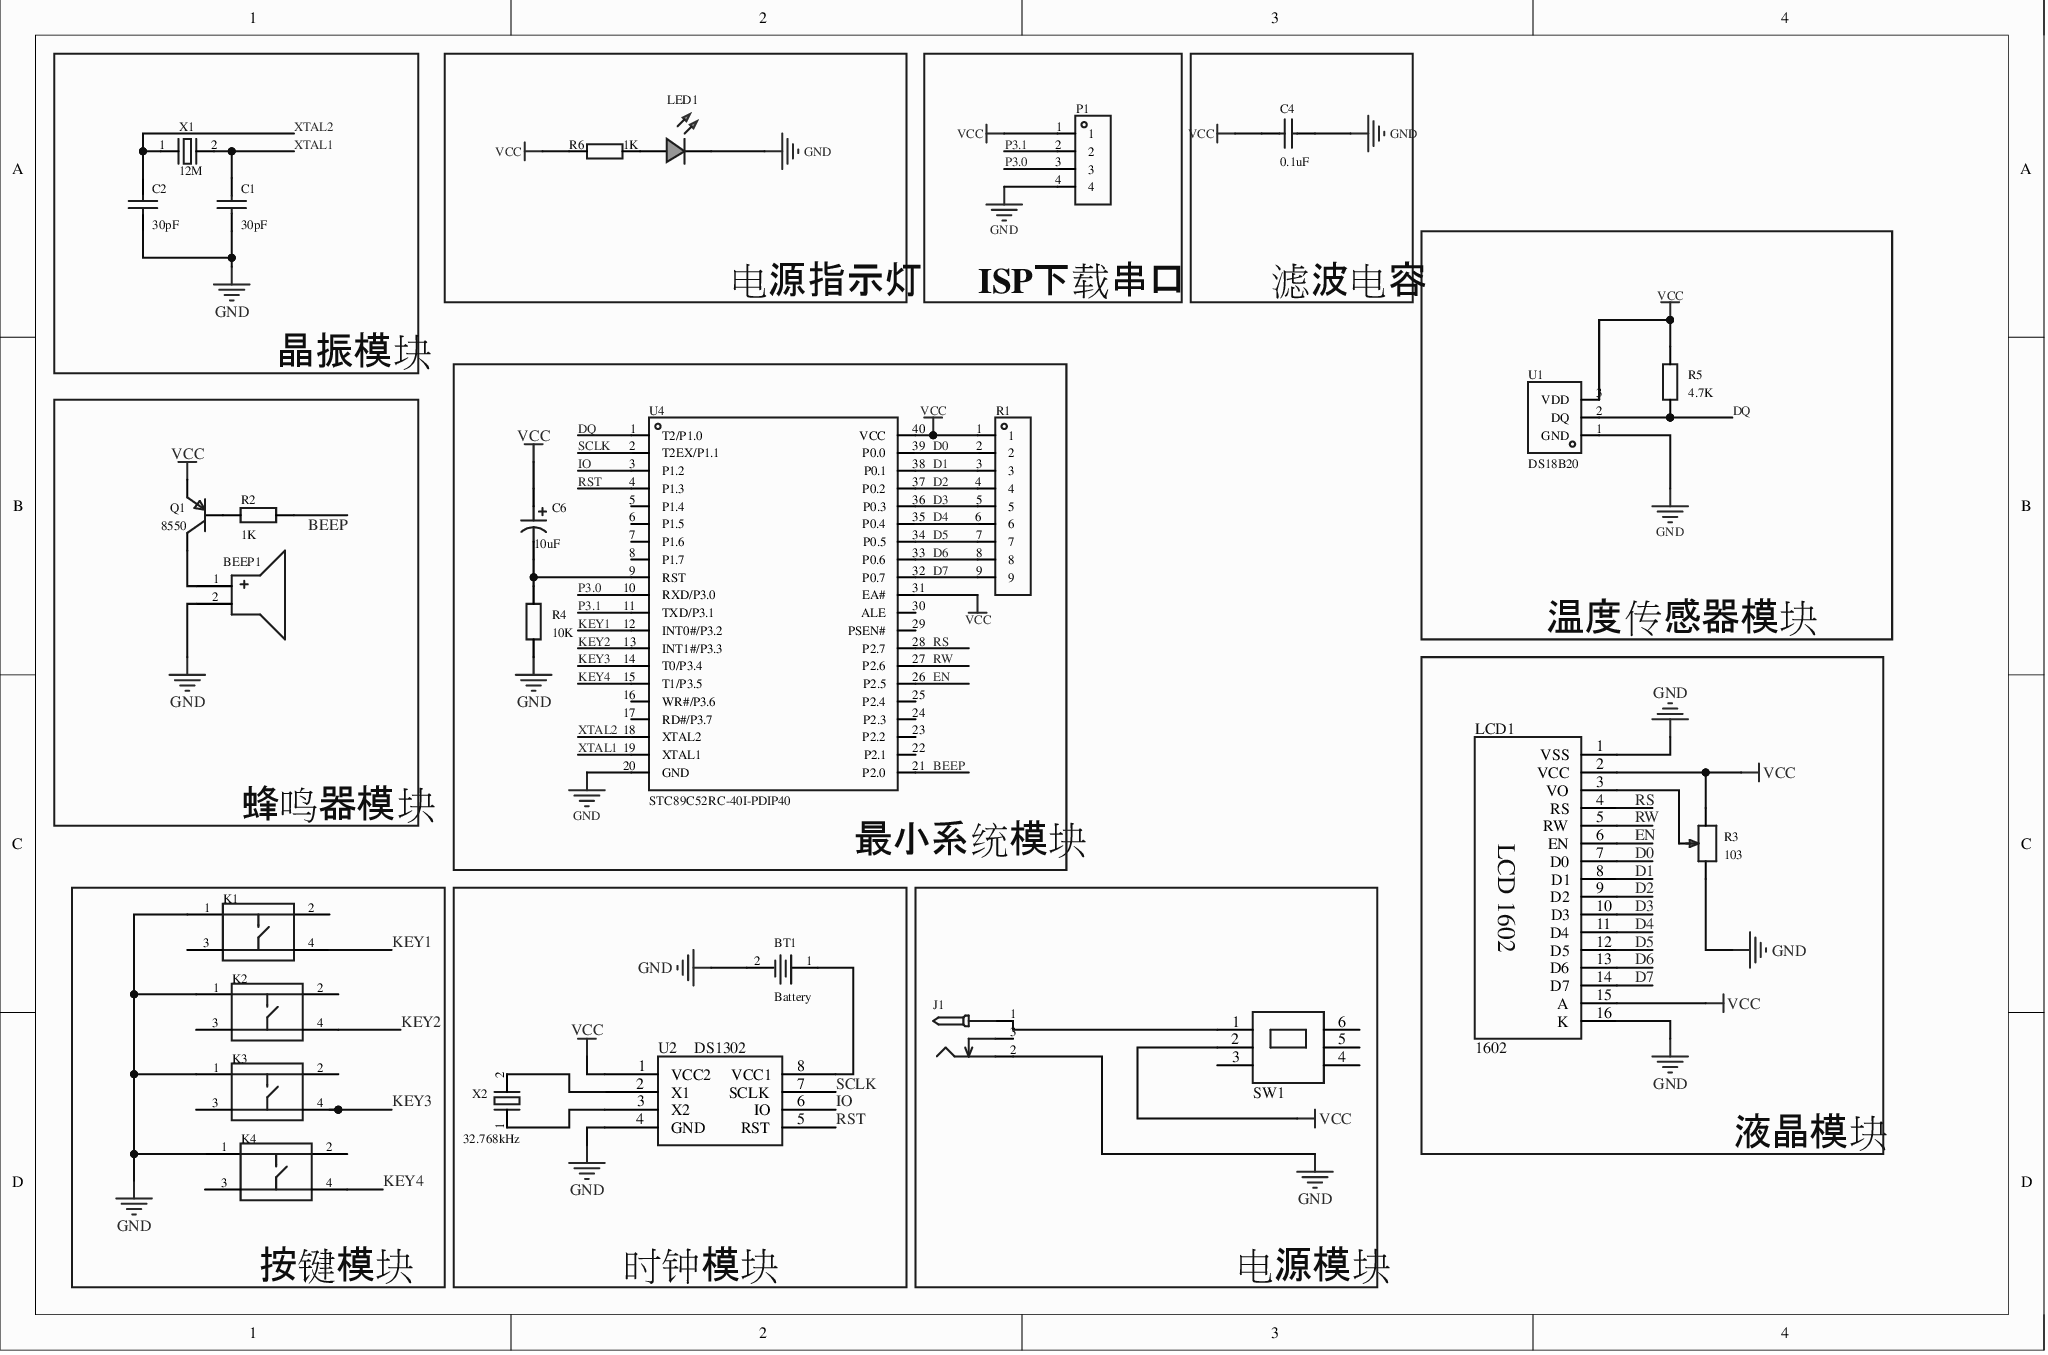
[diagram p0: MISC51236-2.schdoc]
# Altium project MISC51236-3.PrjPcb
1 sheet, 27 parts. Net scope: global (net labels, ports and power ports of the same name join across sheets).
Board file: MISC51236.pcbdoc

## Sheet MISC51236-2.schdoc
size 292 x 193 mm; Name: MISC51236

### Parts
BEEP1  (no value)  [BUZ-TH_BD12.0-P7.60-D0.6-FD]
BT1  Battery  [BAT-TH_CR2032]
C1  30pF  [CAP-TH_L5.0-W4.0-P5.00-D1.0]
C2  30pF  [CAP-TH_L5.0-W4.0-P5.00-D1.0]
C4  0.1uF  [CAP-TH_L5.0-W4.0-P5.00-D1.0]
C6  10uF  [CAP-TH_BD5.0-P2.00-D0.6-FD]
J1  (no value)  [DC-005_2.5]
K1  (no value)  [KEY-TH_4P-L6.0-W6.0-P4.50-LS6.50]
K2  (no value)  [KEY-TH_4P-L6.0-W6.0-P4.50-LS6.50]
K3  (no value)  [KEY-TH_4P-L6.0-W6.0-P4.50-LS6.50]
K4  (no value)  [KEY-TH_4P-L6.0-W6.0-P4.50-LS6.50]
LCD1  1602  [HDR-M-2.54_1X16]
LED1  (no value)  [LED-TH_5mm]
P1  (no value)  [HDR-TH_4P-P2.54-V-M]
Q1  8550  [S8550P_TO-92]
R1  (no value)  [SIP-9_L22.3-W3.2-P2.54_KA2284-SIP-9]
R2  1K  [Res_1/4W]
R3  103  [RES-ADJ-SMD_RM065-V1]
R4  10K  [Res_1/4W]
R5  4.7K  [Res_1/4W]
R6  1K  [Res_1/4W]
SW1  SWT  [SW-TH_6P-L8.5-W8.5-P2.50-LS5.5-BL-2]  (value not drawn)
U1  DS18B20  [TO-92-3_L4.5-W3.5-P1.27-L]
U2  DS1302  [DIP-8_L10.9-W6.4-P2.54-LS7.6-BL]
U4  STC89C52RC-40I-PDIP40  [DIP-40_L52.0-W13.7-P2.54-LS15.2-BL]
X1  12M  [HC-49S_L11.5-W4.7-P4.88]
X2  32.768kHz  [XTAL2]

### Blocks framed on the sheet
晶振模块: C1 C2 X1
电源指示灯: LED1 R6
ISP下载串口: P1
滤波电容: C4
温度传感器模块: R5 U1
最小系统模块: C6 R1 R4 U4
蜂鸣器模块: BEEP1 Q1 R2
液晶模块: LCD1 R3
按键模块: K1-K4
时钟模块: BT1 U2 X2
电源模块: J1 SW1

### Nets
GND: BEEP1.2(-) BT1.2 C1.1 C2.1 C4.2 J1.2 K1.1 K2.1 K3.1 K4.1 LCD1.1(VSS) LCD1.16(K) LED1.2(A) P1.4 R3.1 R4.1 U1.1(GND) U2.4(GND) U4.20(GND)
VCC: C4.1 C6.1 LCD1.2(VCC) LCD1.15(A) P1.1 Q1.1(E) R1.1 R3.3 R5.2 R6.1 SW1.2 U1.3(VDD) U2.1(VCC2) U4.31(EA#) U4.40(VCC)
BEEP: R2.2 U4.21(P2.0)
D0: LCD1.7(D0) R1.2 U4.39(P0.0)
D1: LCD1.8(D1) R1.3 U4.38(P0.1)
D2: LCD1.9(D2) R1.4 U4.37(P0.2)
D3: LCD1.10(D3) R1.5 U4.36(P0.3)
D4: LCD1.11(D4) R1.6 U4.35(P0.4)
D5: LCD1.12(D5) R1.7 U4.34(P0.5)
D6: LCD1.13(D6) R1.8 U4.33(P0.6)
D7: LCD1.14(D7) R1.9 U4.32(P0.7)
DQ: R5.1 U1.2(DQ) U4.1(T2/P1.0)
EN: LCD1.6(EN) U4.26(P2.5)
IO: U2.6(IO) U4.3(P1.2)
KEY1: K1.4 U4.12(INT0#/P3.2)
KEY2: K2.4 U4.13(INT1#/P3.3)
KEY3: K3.4 U4.14(T0/P3.4)
KEY4: K4.4 U4.15(T1/P3.5)
P3.0: P1.3 U4.10(RXD/P3.0)
P3.1: P1.2 U4.11(TXD/P3.1)
RS: LCD1.4(RS) U4.28(P2.7)
RST: U2.5(RST) U4.4(P1.3)
RW: LCD1.5(RW) U4.27(P2.6)
SCLK: U2.7(SCLK) U4.2(T2EX/P1.1)
XTAL1: C1.2 U4.19(XTAL1) X1.2
XTAL2: C2.2 U4.18(XTAL2) X1.1
NetBEEP1_1: BEEP1.1(+) Q1.3(C)
NetBT1_1: BT1.1 U2.8(VCC1)
NetC6_2: C6.2 R4.2 U4.9(RST)
NetJ1_1: J1.1 SW1.1
NetLCD1_3: LCD1.3(VO) R3.2
NetLED1_1: LED1.1(C) R6.2
NetQ1_2: Q1.2(B) R2.1
NetU2_2: U2.2(X1) X2.2
NetU2_3: U2.3(X2) X2.1

Not connected (* = marked no-connect by the designer): J1 3*; K1 2* 3*; K2 2* 3*; K3 2* 3*; K4 2* 3*; SW1 3(2)* 4(3)* 5(4)* 6(5)*; U4 5(P1.4)* 6(P1.5)* 7(P1.6)* 8(P1.7)* 16(WR#/P3.6)* 17(RD#/P3.7)* 22(P2.1)* 23(P2.2)* 24(P2.3)* 25(P2.4)* 29(PSEN#)* 30(ALE)*

### Library data of the parts
BEEP1 = BZ-D12-L7_6: AddInBom: yes; ModelId: 16ab50e14c5b4f2c986c135bdba60e370819f05c4eef4c71ace90d822a990e87; ModelName: BUZ-TH_D12.0-H9.5-P7.60; ModelTransform: 472.44,472.176,0,90,0,0,-0.787,0,-177.165; Symbol: BZ-D12-L7_6; Device: BZ-D12-L7_6; LCSC Part Name: BZ-D12-L7_6; SupplierPart: C9900009978; Supplier Footprint: BUZ-TH; JLCPCB Part Class: Extended Part; Supplier: LCSC; ConvertToPcb: yes; FootprintName: BUZ-TH_BD12.0-P7.60-D0.6-FD
BT1 = Q&J CR2032 20-6*9_C9900112302: AddInBom: yes; ModelId: 2a22c62c6e424c70bca0a6138eddf4b70819f05c4eef4c71ace90d822a990e87; ModelTransform: 814.959,786.69055,0,180,0,0,0,0,-196.85; Symbol: Q&J CR2032 20-6*9; Device: Q&J CR2032 20-6*9_C9900112302; Manufacturer Part: Battery; LCSC Part Name: Q&J CR2032 20-6*9; SupplierPart: C9900112302; Supplier Footprint: BAT-TH_CR2032; JLCPCB Part Class: Extended Part; Supplier: LCSC; ConvertToPcb: yes; FootprintName: BAT-TH_CR2032; ModelName: BAT-TH_CR2032
C1 C2 C4 = 瓷片电容47PF 3KV: 容值:-;额定电压:-;温度系数:-;; Symbol: Ceramic capacitors47PF 3KV; AddInBom: yes; ModelId: 7562e8dfad8b481384451709c5473ca60819f05c4eef4c71ace90d822a990e87; ModelName: CAP-TH_BD5.0-W4.0-P5.08; ModelTransform: 224.49711,157.48,0,0,0,0,0,0,-137.795; Device: 瓷片电容47PF 3KV; LCSC Part Name: 47pF(47R) ±10% 3KV; ManufacturerPart: 瓷片电容47PF 3KV; Supplier Footprint: 插件; JLCPCB Part Class: Extended Part; Supplier: LCSC; ConvertToPcb: yes; FootprintName: CAP-TH_L5.0-W4.0-P5.00-D1.0; Voltage Rated: -; Lead Spacing: -; Temperature Coefficient: -; φD: -; Body Thickness: -
  C1 C2: Value: 30pF
  C4: Value: 0.1uF
C6 = 10uF/25V-C5X11DIP: AddInBom: yes; ModelId: e14933aa819f4e768454ffe1b66cd5400819f05c4eef4c71ace90d822a990e87; ModelTransform: 196.70055,196.77528,0,0,0,0,0.118,0,-137.795; Symbol: 10UF/25V-C5X11DIP; Device: 10uF/25V-C5X11DIP; Manufacturer Part: 10uF; LCSC Part Name: 10uF/25V-C5X11DIP; SupplierPart: C9900003841; Supplier Footprint: CAP-TH_BD5.0-P2.00; JLCPCB Part Class: Extended Part; Supplier: LCSC; ConvertToPcb: yes; FootprintName: CAP-TH_BD5.0-P2.00-D0.6-FD; ModelName: CAP-TH_BD5.0-P2.00-D0.6-FD
J1 = DC-005_2.5: ConvertToPcb: yes; ModelId: f168fe383f964e0ea2af0127ff6ac7b40819f05c4eef4c71ace90d822a990e87; ModelName: DC-IN-TH_DC005; ModelTransform: 366.14,553.15,590.55,90,0,0,137.8,-11.81,-157.48; Symbol: DC-005_2.5; Device: DC-005_2.5; AddInBom: yes; Supplier Footprint: 插件; FootprintName: DC-005_2.5
K1-K4 = K2-1102DP-C4SW-04: 电路结构:单刀单掷;按钮形状:圆形按钮;作用力:2.5N;安装方式:直插;开关长度:6mm;开关宽度:6mm;开关高度:5mm;触点电流:50mA;额定电压:12V;带灯:-;工作寿命:10万次;; Manufacturer: 韩国韩荣; AddInBom: yes; ModelId: b38fea4b2e4e408486f1d54ff7bc5cc00819f05c4eef4c71ace90d822a990e87; ModelTransform: 307.086,236.22,0,0,0,0,0,0,-137.795; Circuit: 单刀单掷; Actuator Style: 圆形按钮; Operating Force: 2.5N; Switch Height: 5mm; Contact Current: 50mA; Voltage Rating: 12V; Life: 10万次; Symbol: K2-1102DP-C4SW-04; Device: K2-1102DP-C4SW-04; LCSC Part Name: 轻触按键开关6*6*5; SupplierPart: C110153; Supplier Footprint: 插件-4P,6x6mm; JLCPCB Part Class: Extended Part; Datasheet: https://item.szlcsc.com/datasheet/K2-1102DP-C4SW-04/111374.html; Supplier: LCSC; ConvertToPcb: yes; FootprintName: KEY-TH_4P-L6.0-W6.0-P4.50-LS6.50; ModelName: KEY-TH_4P-L6.0-W6.0-P4.50-LS6.50; Mounting Type: 直插; Length: 6mm; Width: 6mm; With Lamp: -; Operating Temperature: -25℃~+85℃
LCD1 = 1602_1: AddInBom: yes; Device: 1602_1; DesignItemID: 1602; LibraryName: MANUAL; Symbol: 1602; FootprintName: HDR-M-2.54_1X16
LED1 = LED_TH-G_5mm: ConvertToPcb: yes; ModelId: fe7796f666a04da4b4289311169b45200819f05c4eef4c71ace90d822a990e87; ModelName: LED-TH_BD5.8-P2.54-FD_GREEN-1; ModelTransform: 212.58,227.91,537.36,0,0,0,-7.87,0,-196.85; Symbol: LED_TH-G; Device: LED_TH-G_5mm; AddInBom: yes; Supplier Footprint: 插件; FootprintName: LED-TH_5mm
P1 = HDR-M_2.54_1x4P: Symbol: PZ254V-11-04P; ConvertToPcb: yes; ModelId: 112f4d05e8d64e99ab9a333894bea4f90819f05c4eef4c71ace90d822a990e87; ModelName: HDR-TH_4P-P2.54-M-LI-1X4P; ModelTransform: 399.999,104.7242,0,0,0,0,0,0,-118.11; Device: HDR-M_2.54_1x4P; AddInBom: yes; SupplierPart: C492403; Supplier Footprint: 插件; FootprintName: HDR-TH_4P-P2.54-V-M
Q1 = S8550_TO_PNP: ConvertToPcb: yes; ModelId: aafe8e06f2154e7c93506efd0d6632dd0819f05c4eef4c71ace90d822a990e87; ModelName: TO-92-3_L4.9-W3.7-P1.27-L; ModelTransform: 180.78,141.44,417.3,0,0,0,0,0,-200; Symbol: S8550_TO_PNP; Device: S8550_TO_PNP; AddInBom: yes; Supplier Footprint: TO-92; FootprintName: S8550P_TO-92
R1 = HDR-M_2.54-1x9P: Symbol: PZ254V-11-09P; 3D Model: b5c1e988b3bb4503807579736b357ad00819f05c4eef4c71ace90d822a990e87; 3D Model Transform: 890.15562,98.425,0,0,0,0,0,0,-118.11; ConvertToPcb: yes; ModelName: HDR-TH_9P-P2.54-M-LI-1X9P; Device: HDR-M_2.54-1x9P; Supplier Part: C492408; Supplier Footprint: 插件; AddInBom: yes; FootprintName: SIP-9_L22.3-W3.2-P2.54_KA2284-SIP-9
R2 R4-R6 = Res_AXIAL-1/4W: Symbol: 电阻; 3D Model: 463263665006444ab7a47bd11b0cf9560819f05c4eef4c71ace90d822a990e87; 3D Model Transform: 427.165,94.32816,0,0,0,0,0,0,-196.85; AddInBom: yes; ModelName: RES-TH_BD2.4-L6.3-P10.30-D0.6; Device: Res_AXIAL-1/4W; Supplier Footprint: 轴向引线; ConvertToPcb: yes; FootprintName: Res_1/4W
  R2 R6: Value: 1K
  R4: Value: 10K
  R5: Value: 4.7K
R3 = RM065-V1-103: AddInBom: yes; ModelId: c816c2b7942147f5a832150e8ef6960c0819f05c4eef4c71ace90d822a990e87; ModelTransform: 255.905,283.464,0,0,0,0,0.025,-3.937,-157.48; Symbol: RM065-V1-103; Device: RM065-V1-103; Manufacturer Part: 103; LCSC Part Name: RM065-V1-103; SupplierPart: C54661; Supplier Footprint: -; JLCPCB Part Class: Extended Part; Supplier: LCSC; ConvertToPcb: yes; FootprintName: RES-ADJ-SMD_RM065-V1; ModelName: RES-ADJ-SMD_RM065-V1
SW1 = SWT_1: AddInBom: yes; Device: SWT_1; DesignItemID: SWT; LibraryName: Schlib; Symbol: SWT; FootprintName: SW-TH_6P-L8.5-W8.5-P2.50-LS5.5-BL-2
U1 = DS18B20: 检测温度:-55℃~+125℃;精度:±0.4℃;接口类型:单总线;; Manufacturer: HXY MOSFET(华轩阳电子); Symbol: DS18B20_C5451632; AddInBom: yes; ModelId: 45fa6cddef3743c6aacf8db740a3bc4c0819f05c4eef4c71ace90d822a990e87; ModelTransform: 177.165,137.795,0,0,0,0,0,29.528,-98.425; Tolerance: ±0.4℃; Voltage - Supply: 2.5V~5.5V; Standby Current: 1uA; Interface: 单总线; Temperature Conversion Time: 400ms; Temperature Resolution: 12bit; Device: DS18B20; LCSC Part Name: 温度-10℃~70℃ 精度±0.4℃ 电压2.5V~5.5V; SupplierPart: C5451632; ManufacturerPart: DS18B20; Supplier Footprint: TO-92; JLCPCB Part Class: Extended Part; Datasheet: https://item.szlcsc.com/datasheet/DS18B20/6355375.html; Supplier: LCSC; ConvertToPcb: yes; FootprintName: TO-92-3_L4.5-W3.5-P1.27-L; ModelName: TO-92-3_L4.5-W3.5-P1.27-L; Detection Temperature Range: -55℃~+125℃; Operating Temperature: -
U2 = DS1302: AddInBom: yes; Device: DS1302; DesignItemID: DS1302; LibraryName: MANUAL; Symbol: DS1302; FootprintName: DIP-8_L10.9-W6.4-P2.54-LS7.6-BL
U4 = STC89C52RC-40I-PDIP40: CPU内核:51家族;CPU最大主频:-;; Manufacturer: STC; AddInBom: yes; ModelId: 16d4686a009b4ddca948f91eddb57b140819f05c4eef4c71ace90d822a990e87; ModelName: DIP-40_L52.3-W13.8-H4.0-LS15.24-P2.54; ModelTransform: 2059.051,615.743,0,0,0,0,0,0,-118.11; CPU Core: 51家族; Program Storage Size: 8KB; Program Memory Type: FLASH; Voltage - Supply: 3.3V~5.5V; Symbol: STC89C52RC-40I; Device: STC89C52RC-40I-PDIP40; LCSC Part Name: 单片机原理及应用; SupplierPart: C14022; ManufacturerPart: STC89C52RC-40I-PDIP40; Supplier Footprint: DIP-40; JLCPCB Part Class: Extended Part; Datasheet: https://item.szlcsc.com/datasheet/STC89C52RC-40I-PDIP40/14679.html; Supplier: LCSC; ConvertToPcb: yes; FootprintName: DIP-40_L52.0-W13.7-P2.54-LS15.2-BL; CPU Maximum Speed: -; RAM Size: -; EEPROM: -; Number of I/O: -; ADC (Bit): -; DAC (Bit): -
X1 = SWXSBBCVE0-16.000000: 晶振类型:直插晶振;频率:16MHz;常温频差:±20ppm;负载电容:12pF;频率稳定度:±30ppm;; Manufacturer: Starwave(思大); AddInBom: yes; ModelId: 8681f9edbc4c49baa7439b9863851e5c0819f05c4eef4c71ace90d822a990e87; ModelTransform: 452.755,183.4642,0,0,0,0,0,0,-137.795; Normal temperature Frequency Tolerance: ±20ppm; Load Capacitance: 12pF; Frequency Stability: ±30ppm; Equivalent Series Resistance(ESR): 50Ω; Symbol: SWXSBBCVE0-16.000000; Device: SWXSBBCVE0-16.000000; Value: 12M; LCSC Part Name: 无源晶振; ManufacturerPart: SWXSBBCVE0-16.000000; Supplier Footprint: HC-49S; JLCPCB Part Class: Extended Part; Datasheet: https://item.szlcsc.com/datasheet/SWXSBBCVE0-16.000000/24100442.html; Supplier: LCSC; ConvertToPcb: yes; FootprintName: HC-49S_L11.5-W4.7-P4.88; ModelName: HC-49S_L11.5-W4.7-P4.88; Type: 直插晶振; Operating Temperature: -40℃~+85℃
X2 = AB15T-32.768KHZ: 频率:32.768kHz;常温频差:±20ppm;外接负载电容:12.5pF;频率稳定度(全温):-;; Manufacturer: ABRACON; AddInBom: yes; ModelId: 9fdeeb9d7ef84072bac6c58c302789500819f05c4eef4c71ace90d822a990e87; ModelName: CRYSTAL-TH_BD1.4-P0.45-D0.2; ModelTransform: 55.00706,55.09,0,0,0,0,0,0,-169.291; Normal temperature Frequency Tolerance: ±20ppm; External load capacitor: 12.5pF; Equivalent Series Resistance (ESR): 40kΩ; Symbol: AB15T-32.768KHZ; Device: AB15T-32.768KHZ; LCSC Part Name: 32.768kHz ±20ppm 12.5pF; SupplierPart: C1669866; ManufacturerPart: AB15T-32.768KHZ; Supplier Footprint: DT-15; JLCPCB Part Class: Extended Part; Datasheet: https://atta.szlcsc.com/upload/public/pdf/source/20210504/0EA8EED362197519A7C3815AD65C577B.pdf; Supplier: LCSC; ConvertToPcb: yes; FootprintName: XTAL2; Value: 32.768kHz; Frequency Stability(Full temperature range): -; Operating Temperature: -20℃~+70℃